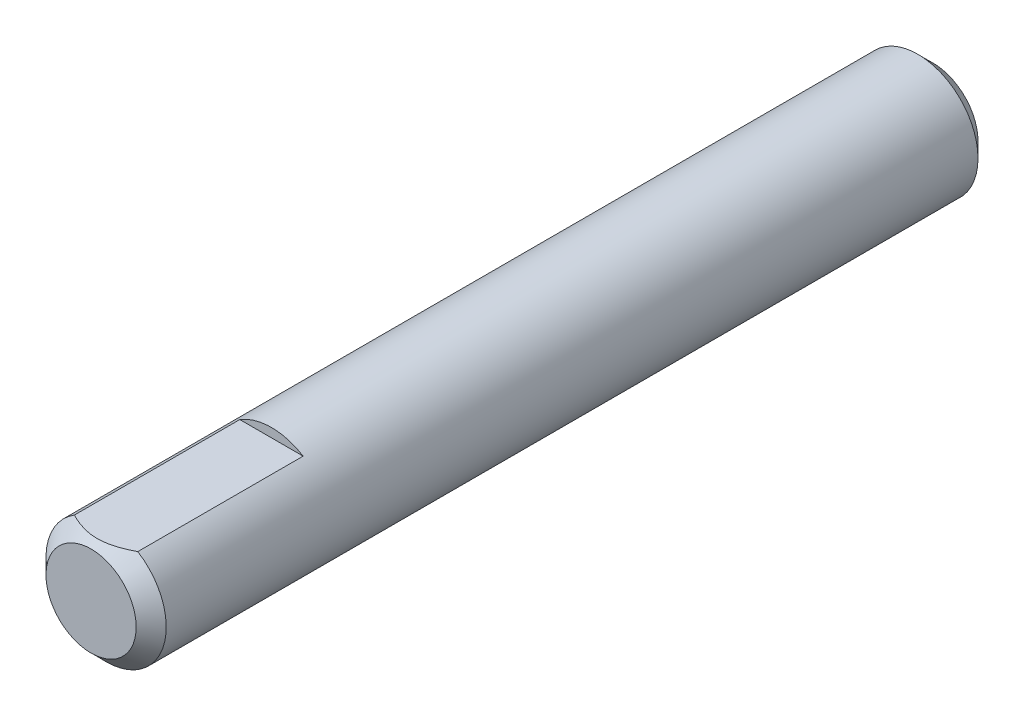
from build123d import *

# Parameters (mm, degrees)
SKETCH1_R           = 2
BOSS_EXTRUDE1_DEPTH = 28
CHAMFER1_SIZE       = 0.5
SKETCH3_W           = 9.979897522
SKETCH3_H           = 2.201799933
CUT_EXTRUDE1_DEPTH  = 6


with BuildPart() as part:
    # Sketch1 → Boss-Extrude1 (new body)
    with BuildSketch(Plane.XY):
        Circle(SKETCH1_R)
    extrude(amount=BOSS_EXTRUDE1_DEPTH)

    # Chamfer1
    chamfer1_edges = [part.edges().sort_by_distance(p)[0] for p in [
        (-2, 0, 0),
        (-2, 0, 28),
    ]]
    chamfer(chamfer1_edges, length=CHAMFER1_SIZE)

    # Sketch3 → Cut-Extrude1 (cut)
    with BuildSketch(Plane.XY.offset(28)):
        with Locations((0.02893888, 2.800899967)):
            Rectangle(SKETCH3_W, SKETCH3_H)
    extrude(amount=-CUT_EXTRUDE1_DEPTH, mode=Mode.SUBTRACT)


solid = part.part
